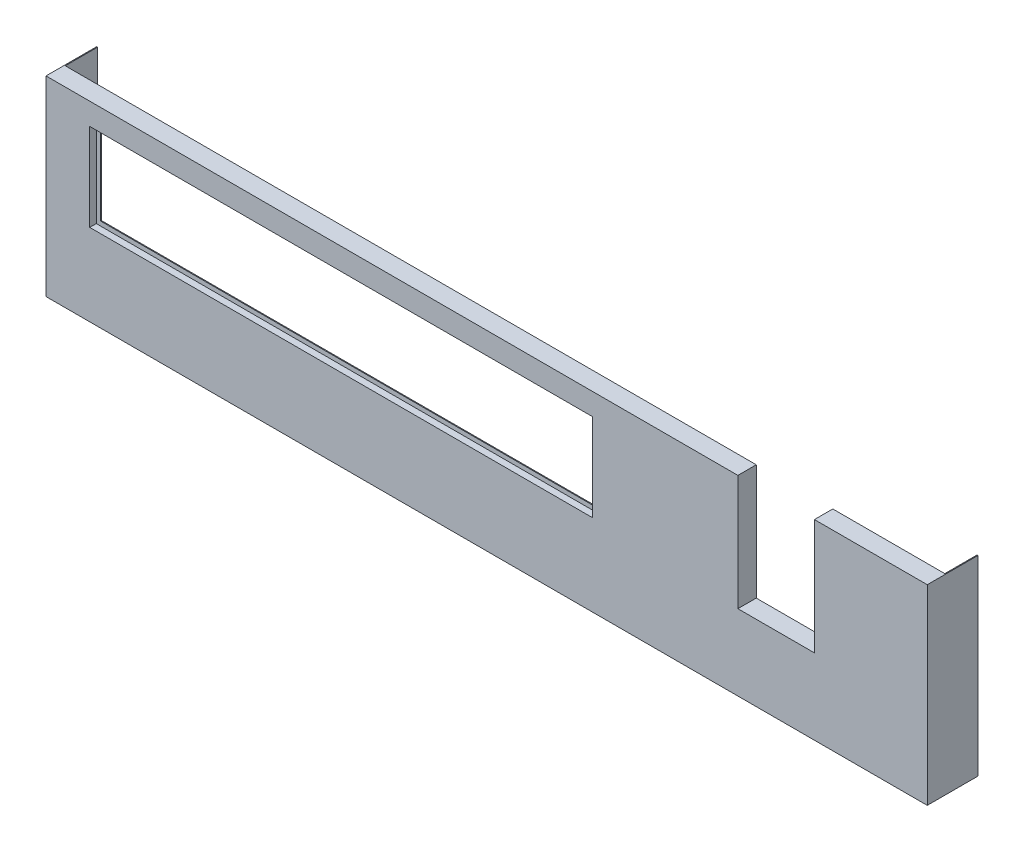
SolidWorks part; units mm, degrees
ref_plane "前视基准面" through (0, 0, 0) normal (0, 0, 1) x (1, 0, 0)
ref_plane "上视基准面" through (0, 0, 0) normal (0, 1, 0) x (1, 0, 0)
ref_plane "右视基准面" through (0, 0, 0) normal (1, 0, 0) x (0, 0, -1)
sketch "草图2" plane through (0, 0, 0) normal (0, 0, 1) x (1, 0, 0)
  line L0 (1757, 437) -> (2015, 437)
  line L1 (0, 0) -> (2015, 0)
  line L2 (0, 0) -> (0, 437)
  line L3 (0, 437) -> (1582, 437)
  line L4 (2015, 0) -> (2015, 437)
  line L6 (1582, 437) -> (1582, 173)
  line L7 (1582, 173) -> (1757, 173)
  line L8 (1757, 437) -> (1757, 173)
  dimension "D1" = 437
  dimension "D2" = 2015
  dimension "D3" = 175
  dimension "D4" = 258
  dimension "D5" = 264
extrude "凸台-拉伸1" add sketch "草图2" along normal blind 2
sketch "草图7" plane through (0, 0, 0) normal (0, 0, -1) x (-1, 0, 0)
  line L1 (-2013, 437) -> (-2015, 437)
  line L2 (-2013, 0) -> (-2013, 437)
  line L3 (-2013, 0) -> (-2013, 437)
  line L4 (-2015, 437) -> (-2015, 0)
  line L5 (-2015, 0) -> (-2013, 0)
  dimension "D1" = 2
extrude "凸台-拉伸2" add sketch "草图7" along normal blind 114
sketch "草图8" plane through (0, 0, 0) normal (0, 0, -1) x (-1, 0, 0)
  line L0 (0, 0) -> (-2013, 0) construction
  line L1 (0, 437) -> (-2, 437)
  line L2 (0, 437) -> (0, 0)
  line L3 (0, 0) -> (-2, 0)
  line L4 (-2, 437) -> (-2, 0)
  dimension "D1" = 2
extrude "凸台-拉伸3" add sketch "草图8" along normal blind 114
sketch "草图9" plane through (0, 0, 0) normal (0, 0, -1) x (-1, 0, 0)
  line L15 (-2013, 435) -> (-1759, 435)
  line L16 (-1759, 435) -> (-1759, 171)
  line L17 (-1759, 171) -> (-1580, 171)
  line L18 (-1580, 171) -> (-1580, 435)
  line L19 (-1580, 435) -> (-2, 435)
  line L20 (-1582, 437) -> (-2, 437)
  line L21 (-1582, 173) -> (-1582, 437)
  line L22 (-1757, 173) -> (-1582, 173)
  line L23 (-1757, 437) -> (-1757, 173)
  line L24 (-2013, 437) -> (-1757, 437)
  line L25 (-1582, 437) -> (-2, 437)
  line L26 (-1582, 173) -> (-1582, 437)
  line L27 (-1757, 173) -> (-1582, 173)
  line L28 (-1757, 437) -> (-1757, 173)
  line L29 (-2013, 437) -> (-1757, 437)
  line L30 (-2013, 437) -> (-2013, 435)
  line L31 (-2, 437) -> (-2, 435)
  dimension "D1" = 0
  dimension "D2" = 2
extrude "凸台-拉伸4" add sketch "草图9" along normal blind 40
sketch "草图10" plane through (0, 0, 2) normal (0, 0, 1) x (1, 0, 0)
  line L0 (1582, 437) -> (0, 437) construction
  line L1 (100, 387) -> (1250, 387)
  line L2 (100, 387) -> (100, 187)
  line L3 (100, 187) -> (1250, 187)
  line L4 (1250, 387) -> (1250, 187)
  line L5 (0, 437) -> (0, 0) construction
  dimension "D1" = 50
  dimension "D2" = 100
  dimension "D3" = 1150
  dimension "D4" = 200
extrude "切除-拉伸1" cut sketch "草图10" against normal blind 10
sketch "草图11" plane through (0, 0, 0) normal (0, -1, 0) x (1, 0, 0)
  line L0 (2015, 2) -> (2015, -114) construction
  line L1 (0, 2) -> (2015, 2)
  line L2 (0, 2) -> (0, -40.4679)
  line L3 (0, -40.4679) -> (2015, -40.4679)
  line L4 (2015, 2) -> (2015, -40.4679)
extrude "凸台-拉伸5" add sketch "草图11" against normal blind 2
sketch "草图12" plane through (0, 0, 0) normal (0, 0, -1) x (-1, 0, 0)
  line L10 (-1252, 389) -> (-1252, 185)
  line L11 (-1252, 185) -> (-98, 185)
  line L12 (-98, 185) -> (-98, 389)
  line L13 (-98, 389) -> (-1252, 389)
  line L14 (-100, 187) -> (-100, 387)
  line L15 (-1250, 187) -> (-100, 187)
  line L16 (-100, 387) -> (-1250, 387)
  line L17 (-1250, 387) -> (-1250, 187)
  line L18 (-100, 187) -> (-100, 387)
  line L19 (-1250, 187) -> (-100, 187)
  line L20 (-100, 387) -> (-1250, 387)
  line L21 (-1250, 387) -> (-1250, 187)
  dimension "D1" = 0
  dimension "D2" = 2
extrude "凸台-拉伸6" add sketch "草图12" along normal blind 15
sketch "草图13" plane through (0, 0, -15) normal (0, 0, -1) x (-1, 0, 0)
  line L0 (-1252, 185) -> (-98, 185) construction
  line L1 (-1252, 389) -> (-98, 389)
  line L2 (-1252, 389) -> (-1252, 185)
  line L3 (-1252, 185) -> (-98, 185)
  line L4 (-98, 389) -> (-98, 185)
  line L5 (-1252, 185) -> (-98, 185) construction
  line L16 (-98, 185) -> (-98, 389) construction
  line L20 (-1240, 377) -> (-1240, 197)
  line L21 (-110, 377) -> (-1240, 377)
  line L22 (-1240, 197) -> (-110, 197)
  line L23 (-110, 197) -> (-110, 377)
  line L24 (-1240, 377) -> (-1240, 197)
  line L25 (-110, 377) -> (-1240, 377)
  line L26 (-1240, 197) -> (-110, 197)
  line L27 (-110, 197) -> (-110, 377)
  dimension "D1" = 10
extrude "凸台-拉伸7" add sketch "草图13" against normal blind 2
